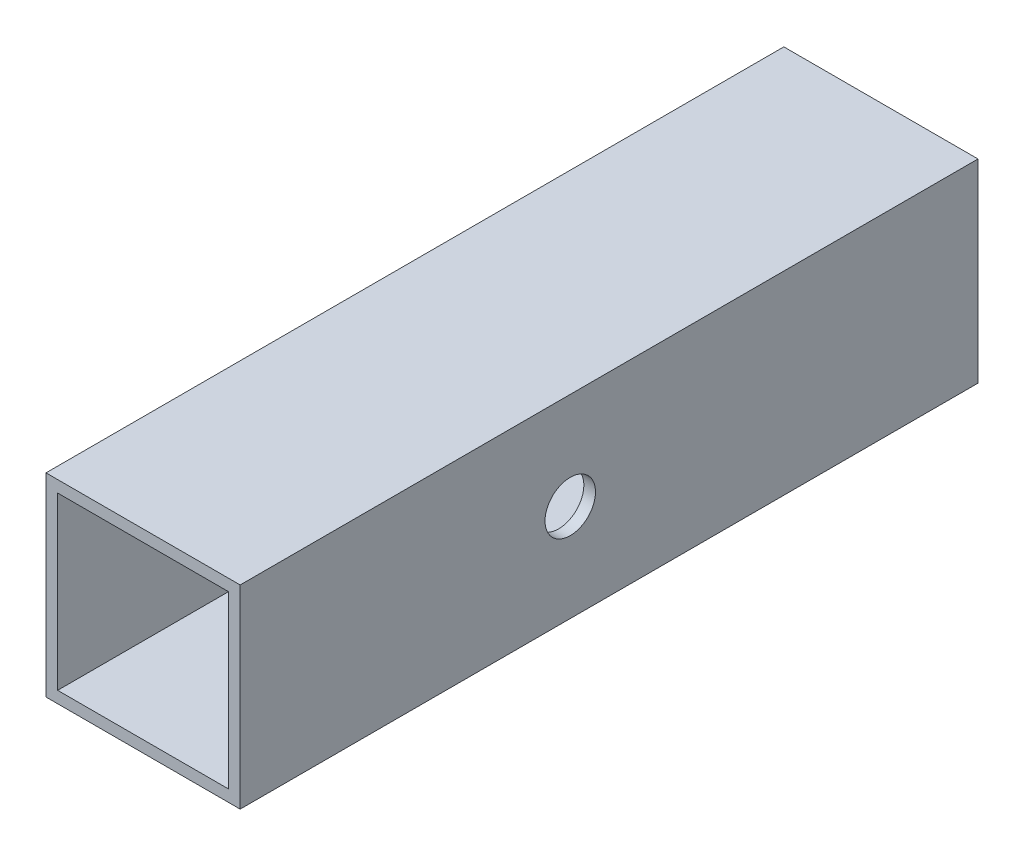
SolidWorks part; units mm, degrees
ref_plane "前视基准面" through (0, 0, 0) normal (0, 0, 1) x (1, 0, 0)
ref_plane "上视基准面" through (0, 0, 0) normal (0, 1, 0) x (1, 0, 0)
ref_plane "右视基准面" through (0, 0, 0) normal (1, 0, 0) x (0, 0, -1)
sketch "草图1" plane through (0, 0, 0) normal (0, 0, 1) x (1, 0, 0)
  line L0 (0, 0) -> (50, 0)
  line L1 (50, 0) -> (50, -50)
  line L2 (50, -50) -> (0, -50)
  line L3 (0, -50) -> (0, 0)
  line L4 (3, -3) -> (47, -3)
  line L5 (47, -3) -> (47, -47)
  line L6 (47, -47) -> (3, -47)
  line L7 (3, -47) -> (3, -3)
  dimension "D1" = 3
extrude "凸台-拉伸2" add sketch "草图1" along normal blind 190
sketch "草图4" plane through (50, 0, 0) normal (1, 0, 0) x (0, 0, -1)
  line L0 (-190, -25) -> (0, -25)
  line L1 (-190, -50) -> (-190, 0) construction
  line L2 (0, -50) -> (0, 0) construction
sketch "草图5" plane through (50, 0, 0) normal (1, 0, 0) x (0, 0, -1)
  circle A0 centre (-105, -25) radius 6.5
  circle A1 centre (-324.8394, -25) radius 6.5
extrude "切除-拉伸1" cut sketch "草图5" against normal blind 130
